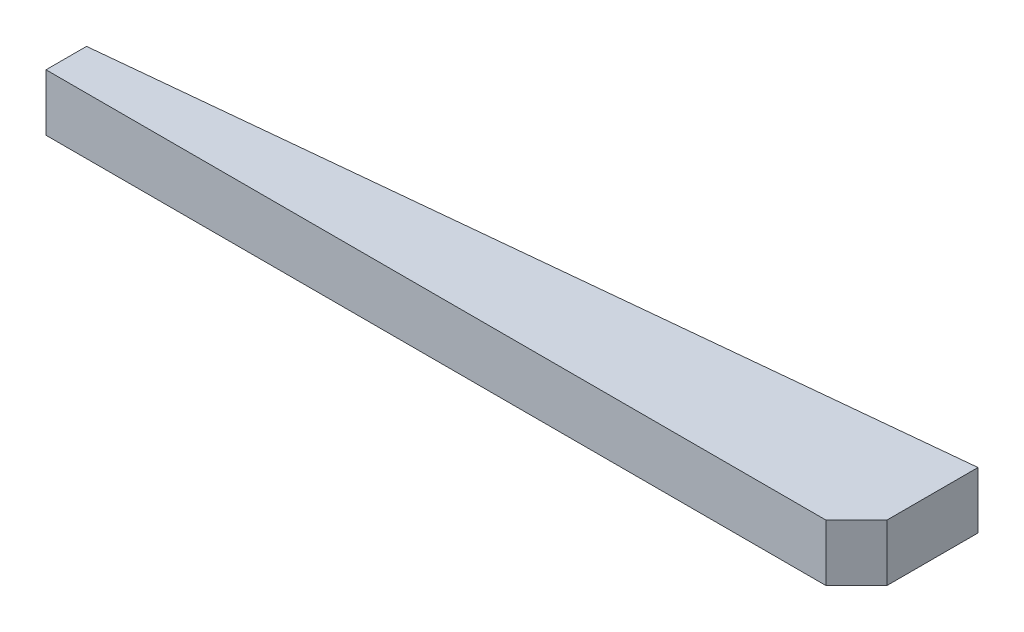
from build123d import *

# Parameters (mm, degrees)
BOSS_EXTRUDE1_DEPTH = 28


with BuildPart() as part:
    # Sketch1 → Boss-Extrude1 (new body)
    with BuildSketch(Plane(origin=(0, 0, 0), x_dir=(1, 0, 0), z_dir=(0, 1, 0))):
        Polygon((2011.523887052, 1584.007884982), (2396.523887052, 1584.007884982), (2411.523887052, 1599.007884982), (2411.523887052, 1644.007884982), (2011.523887052, 1604.007884982), align=None)
    extrude(amount=BOSS_EXTRUDE1_DEPTH)


solid = part.part
